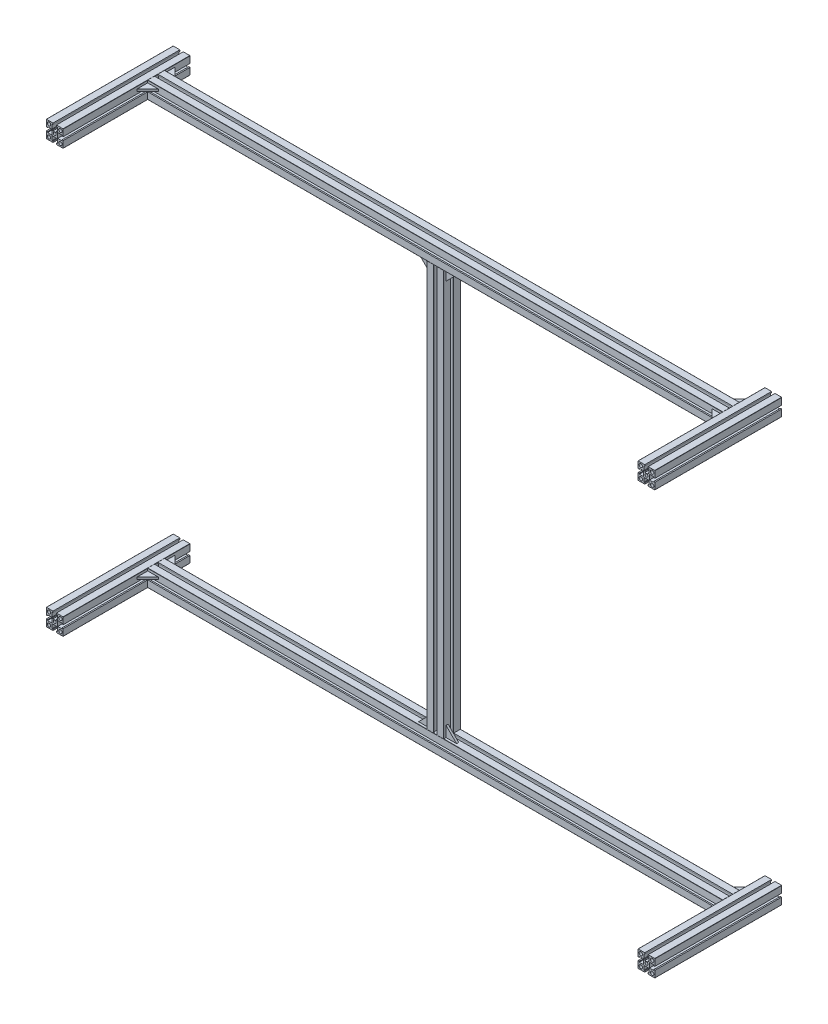
from build123d import *

# Parameters (mm, degrees)
SKETCH1_R                    = 3.4
SKETCH1_R_2                  = 4
F_40_X_40GF_X_R0_5_3_DEPTH   = 300
SKETCH1_ON_SEGMENT_2_R       = 3.4
SKETCH1_ON_SEGMENT_2_R_2     = 4
F_40_X_40GF_X_R0_5_3_2_DEPTH = 300
SKETCH1_ON_SEGMENT_3_R       = 3.4
SKETCH1_ON_SEGMENT_3_R_2     = 4
F_40_X_40GF_X_R0_5_3_3_DEPTH = 300
SKETCH1_ON_SEGMENT_4_R       = 3.4
SKETCH1_ON_SEGMENT_4_R_2     = 4
F_40_X_40GF_X_R0_5_3_4_DEPTH = 300
SKETCH1_ON_SEGMENT_5_R       = 3.4
SKETCH1_ON_SEGMENT_5_R_2     = 4
F_40_X_40GF_X_R0_5_3_5_DEPTH = 1402
SKETCH1_ON_SEGMENT_6_R       = 3.4
SKETCH1_ON_SEGMENT_6_R_2     = 4
F_40_X_40GF_X_R0_5_3_6_DEPTH = 1402
SKETCH1_ON_SEGMENT_7_R       = 3.4
SKETCH1_ON_SEGMENT_7_R_2     = 4
F_40_X_40GF_X_R0_5_3_7_DEPTH = 1002
GUSSET_2_THICKNESS           = 5
GUSSET_3_THICKNESS           = 5
GUSSET_4_THICKNESS           = 5
GUSSET_5_THICKNESS           = 5
GUSSET_6_THICKNESS           = 5
GUSSET_7_THICKNESS           = 5
GUSSET_8_THICKNESS           = 5
GUSSET_9_THICKNESS           = 5
GUSSET_12_THICKNESS          = 5
GUSSET_13_THICKNESS          = 5
GUSSET_14_THICKNESS          = 5
GUSSET_15_THICKNESS          = 5


with BuildPart() as part:
    # Sketch1 → 铝型材 40 X 40GF X R0.5(3) (new body)
    with BuildSketch(Plane(origin=(-700, 500, 0), x_dir=(1, 0, 0), z_dir=(0, 0, 1))):
        with BuildLine():
            Line((-19.5, 20), (-4, 20))
            Line((-4, 20), (-4, 17))
            Line((-4, 17), (-6, 17))
            Line((-6, 17), (-6, 7))
            Line((-6, 7), (-4, 7))
            Line((-4, 7), (-4, 4))
            Line((-4, 4), (4, 4))
            Line((4, 4), (4, 7))
            Line((4, 7), (6, 7))
            Line((6, 7), (6, 17))
            Line((6, 17), (4, 17))
            Line((4, 17), (4, 20))
            Line((4, 20), (19.5, 20))
            ThreePointArc((19.5, 20), (19.853553391, 19.853553391), (20, 19.5))
            Line((20, 19.5), (20, 4))
            Line((20, 4), (17, 4))
            Line((17, 4), (17, 6))
            Line((17, 6), (7, 6))
            Line((7, 6), (7, -6))
            Line((7, -6), (17, -6))
            Line((17, -6), (17, -4))
            Line((17, -4), (20, -4))
            Line((20, -4), (20, -19.5))
            ThreePointArc((20, -19.5), (19.853553391, -19.853553391), (19.5, -20))
            Line((19.5, -20), (4, -20))
            Line((4, -20), (4, -17))
            Line((4, -17), (6, -17))
            Line((6, -17), (6, -7))
            Line((6, -7), (-6, -7))
            Line((-6, -7), (-6, -17))
            Line((-6, -17), (-4, -17))
            Line((-4, -17), (-4, -20))
            Line((-4, -20), (-19.5, -20))
            ThreePointArc((-19.5, -20), (-19.853553391, -19.853553391), (-20, -19.5))
            Line((-20, -19.5), (-20, -4))
            Line((-20, -4), (-17, -4))
            Line((-17, -4), (-17, -6))
            Line((-17, -6), (-7, -6))
            Line((-7, -6), (-7, 6))
            Line((-7, 6), (-17, 6))
            Line((-17, 6), (-17, 4))
            Line((-17, 4), (-20, 4))
            Line((-20, 4), (-20, 19.5))
            ThreePointArc((-20, 19.5), (-19.853553391, 19.853553391), (-19.5, 20))
        make_face()
        Circle(SKETCH1_R, mode=Mode.SUBTRACT)
        with Locations((-13.435028843, 13.435028843)):
            Circle(SKETCH1_R_2, mode=Mode.SUBTRACT)
        with Locations((13.435028843, 13.435028843)):
            Circle(SKETCH1_R_2, mode=Mode.SUBTRACT)
        with Locations((13.435028843, -13.435028843)):
            Circle(SKETCH1_R_2, mode=Mode.SUBTRACT)
        with Locations((-13.435028843, -13.435028843)):
            Circle(SKETCH1_R_2, mode=Mode.SUBTRACT)
    extrude(amount=F_40_X_40GF_X_R0_5_3_DEPTH)


with BuildPart() as body_2:
    # Sketch1 on segment 2 (carried to segment 2) → 40 X 40GF X R0.5_3 2 (new body)
    with BuildSketch(Plane(origin=(700, 500, 0), x_dir=(1, 0, 0), z_dir=(0, 0, 1))):
        with BuildLine():
            Line((-19.5, 20), (-4, 20))
            Line((-4, 20), (-4, 17))
            Line((-4, 17), (-6, 17))
            Line((-6, 17), (-6, 7))
            Line((-6, 7), (-4, 7))
            Line((-4, 7), (-4, 4))
            Line((-4, 4), (4, 4))
            Line((4, 4), (4, 7))
            Line((4, 7), (6, 7))
            Line((6, 7), (6, 17))
            Line((6, 17), (4, 17))
            Line((4, 17), (4, 20))
            Line((4, 20), (19.5, 20))
            ThreePointArc((19.5, 20), (19.853553391, 19.853553391), (20, 19.5))
            Line((20, 19.5), (20, 4))
            Line((20, 4), (17, 4))
            Line((17, 4), (17, 6))
            Line((17, 6), (7, 6))
            Line((7, 6), (7, -6))
            Line((7, -6), (17, -6))
            Line((17, -6), (17, -4))
            Line((17, -4), (20, -4))
            Line((20, -4), (20, -19.5))
            ThreePointArc((20, -19.5), (19.853553391, -19.853553391), (19.5, -20))
            Line((19.5, -20), (4, -20))
            Line((4, -20), (4, -17))
            Line((4, -17), (6, -17))
            Line((6, -17), (6, -7))
            Line((6, -7), (-6, -7))
            Line((-6, -7), (-6, -17))
            Line((-6, -17), (-4, -17))
            Line((-4, -17), (-4, -20))
            Line((-4, -20), (-19.5, -20))
            ThreePointArc((-19.5, -20), (-19.853553391, -19.853553391), (-20, -19.5))
            Line((-20, -19.5), (-20, -4))
            Line((-20, -4), (-17, -4))
            Line((-17, -4), (-17, -6))
            Line((-17, -6), (-7, -6))
            Line((-7, -6), (-7, 6))
            Line((-7, 6), (-17, 6))
            Line((-17, 6), (-17, 4))
            Line((-17, 4), (-20, 4))
            Line((-20, 4), (-20, 19.5))
            ThreePointArc((-20, 19.5), (-19.853553391, 19.853553391), (-19.5, 20))
        make_face()
        Circle(SKETCH1_ON_SEGMENT_2_R, mode=Mode.SUBTRACT)
        with Locations((-13.435028843, 13.435028843)):
            Circle(SKETCH1_ON_SEGMENT_2_R_2, mode=Mode.SUBTRACT)
        with Locations((13.435028843, 13.435028843)):
            Circle(SKETCH1_ON_SEGMENT_2_R_2, mode=Mode.SUBTRACT)
        with Locations((13.435028843, -13.435028843)):
            Circle(SKETCH1_ON_SEGMENT_2_R_2, mode=Mode.SUBTRACT)
        with Locations((-13.435028843, -13.435028843)):
            Circle(SKETCH1_ON_SEGMENT_2_R_2, mode=Mode.SUBTRACT)
    extrude(amount=F_40_X_40GF_X_R0_5_3_2_DEPTH)


with BuildPart() as body_3:
    # Sketch1 on segment 3 (carried to segment 3) → 40 X 40GF X R0.5_3 3 (new body)
    with BuildSketch(Plane(origin=(700, -500, 0), x_dir=(1, 0, 0), z_dir=(0, 0, 1))):
        with BuildLine():
            Line((-19.5, 20), (-4, 20))
            Line((-4, 20), (-4, 17))
            Line((-4, 17), (-6, 17))
            Line((-6, 17), (-6, 7))
            Line((-6, 7), (-4, 7))
            Line((-4, 7), (-4, 4))
            Line((-4, 4), (4, 4))
            Line((4, 4), (4, 7))
            Line((4, 7), (6, 7))
            Line((6, 7), (6, 17))
            Line((6, 17), (4, 17))
            Line((4, 17), (4, 20))
            Line((4, 20), (19.5, 20))
            ThreePointArc((19.5, 20), (19.853553391, 19.853553391), (20, 19.5))
            Line((20, 19.5), (20, 4))
            Line((20, 4), (17, 4))
            Line((17, 4), (17, 6))
            Line((17, 6), (7, 6))
            Line((7, 6), (7, -6))
            Line((7, -6), (17, -6))
            Line((17, -6), (17, -4))
            Line((17, -4), (20, -4))
            Line((20, -4), (20, -19.5))
            ThreePointArc((20, -19.5), (19.853553391, -19.853553391), (19.5, -20))
            Line((19.5, -20), (4, -20))
            Line((4, -20), (4, -17))
            Line((4, -17), (6, -17))
            Line((6, -17), (6, -7))
            Line((6, -7), (-6, -7))
            Line((-6, -7), (-6, -17))
            Line((-6, -17), (-4, -17))
            Line((-4, -17), (-4, -20))
            Line((-4, -20), (-19.5, -20))
            ThreePointArc((-19.5, -20), (-19.853553391, -19.853553391), (-20, -19.5))
            Line((-20, -19.5), (-20, -4))
            Line((-20, -4), (-17, -4))
            Line((-17, -4), (-17, -6))
            Line((-17, -6), (-7, -6))
            Line((-7, -6), (-7, 6))
            Line((-7, 6), (-17, 6))
            Line((-17, 6), (-17, 4))
            Line((-17, 4), (-20, 4))
            Line((-20, 4), (-20, 19.5))
            ThreePointArc((-20, 19.5), (-19.853553391, 19.853553391), (-19.5, 20))
        make_face()
        Circle(SKETCH1_ON_SEGMENT_3_R, mode=Mode.SUBTRACT)
        with Locations((-13.435028843, 13.435028843)):
            Circle(SKETCH1_ON_SEGMENT_3_R_2, mode=Mode.SUBTRACT)
        with Locations((13.435028843, 13.435028843)):
            Circle(SKETCH1_ON_SEGMENT_3_R_2, mode=Mode.SUBTRACT)
        with Locations((13.435028843, -13.435028843)):
            Circle(SKETCH1_ON_SEGMENT_3_R_2, mode=Mode.SUBTRACT)
        with Locations((-13.435028843, -13.435028843)):
            Circle(SKETCH1_ON_SEGMENT_3_R_2, mode=Mode.SUBTRACT)
    extrude(amount=F_40_X_40GF_X_R0_5_3_3_DEPTH)


with BuildPart() as body_4:
    # Sketch1 on segment 4 (carried to segment 4) → 40 X 40GF X R0.5_3 4 (new body)
    with BuildSketch(Plane(origin=(-700, -500, 0), x_dir=(1, 0, 0), z_dir=(0, 0, 1))):
        with BuildLine():
            Line((-19.5, 20), (-4, 20))
            Line((-4, 20), (-4, 17))
            Line((-4, 17), (-6, 17))
            Line((-6, 17), (-6, 7))
            Line((-6, 7), (-4, 7))
            Line((-4, 7), (-4, 4))
            Line((-4, 4), (4, 4))
            Line((4, 4), (4, 7))
            Line((4, 7), (6, 7))
            Line((6, 7), (6, 17))
            Line((6, 17), (4, 17))
            Line((4, 17), (4, 20))
            Line((4, 20), (19.5, 20))
            ThreePointArc((19.5, 20), (19.853553391, 19.853553391), (20, 19.5))
            Line((20, 19.5), (20, 4))
            Line((20, 4), (17, 4))
            Line((17, 4), (17, 6))
            Line((17, 6), (7, 6))
            Line((7, 6), (7, -6))
            Line((7, -6), (17, -6))
            Line((17, -6), (17, -4))
            Line((17, -4), (20, -4))
            Line((20, -4), (20, -19.5))
            ThreePointArc((20, -19.5), (19.853553391, -19.853553391), (19.5, -20))
            Line((19.5, -20), (4, -20))
            Line((4, -20), (4, -17))
            Line((4, -17), (6, -17))
            Line((6, -17), (6, -7))
            Line((6, -7), (-6, -7))
            Line((-6, -7), (-6, -17))
            Line((-6, -17), (-4, -17))
            Line((-4, -17), (-4, -20))
            Line((-4, -20), (-19.5, -20))
            ThreePointArc((-19.5, -20), (-19.853553391, -19.853553391), (-20, -19.5))
            Line((-20, -19.5), (-20, -4))
            Line((-20, -4), (-17, -4))
            Line((-17, -4), (-17, -6))
            Line((-17, -6), (-7, -6))
            Line((-7, -6), (-7, 6))
            Line((-7, 6), (-17, 6))
            Line((-17, 6), (-17, 4))
            Line((-17, 4), (-20, 4))
            Line((-20, 4), (-20, 19.5))
            ThreePointArc((-20, 19.5), (-19.853553391, 19.853553391), (-19.5, 20))
        make_face()
        Circle(SKETCH1_ON_SEGMENT_4_R, mode=Mode.SUBTRACT)
        with Locations((-13.435028843, 13.435028843)):
            Circle(SKETCH1_ON_SEGMENT_4_R_2, mode=Mode.SUBTRACT)
        with Locations((13.435028843, 13.435028843)):
            Circle(SKETCH1_ON_SEGMENT_4_R_2, mode=Mode.SUBTRACT)
        with Locations((13.435028843, -13.435028843)):
            Circle(SKETCH1_ON_SEGMENT_4_R_2, mode=Mode.SUBTRACT)
        with Locations((-13.435028843, -13.435028843)):
            Circle(SKETCH1_ON_SEGMENT_4_R_2, mode=Mode.SUBTRACT)
    extrude(amount=F_40_X_40GF_X_R0_5_3_4_DEPTH)


with BuildPart() as body_5:
    # Sketch1 on segment 5 (carried to segment 5) → 40 X 40GF X R0.5_3 5 (new body)
    with BuildSketch(Plane(origin=(-701, 500, 80), x_dir=(0, 0, -1), z_dir=(1, 0, 0))):
        with BuildLine():
            Line((-19.5, 20), (-4, 20))
            Line((-4, 20), (-4, 17))
            Line((-4, 17), (-6, 17))
            Line((-6, 17), (-6, 7))
            Line((-6, 7), (-4, 7))
            Line((-4, 7), (-4, 4))
            Line((-4, 4), (4, 4))
            Line((4, 4), (4, 7))
            Line((4, 7), (6, 7))
            Line((6, 7), (6, 17))
            Line((6, 17), (4, 17))
            Line((4, 17), (4, 20))
            Line((4, 20), (19.5, 20))
            ThreePointArc((19.5, 20), (19.853553391, 19.853553391), (20, 19.5))
            Line((20, 19.5), (20, 4))
            Line((20, 4), (17, 4))
            Line((17, 4), (17, 6))
            Line((17, 6), (7, 6))
            Line((7, 6), (7, -6))
            Line((7, -6), (17, -6))
            Line((17, -6), (17, -4))
            Line((17, -4), (20, -4))
            Line((20, -4), (20, -19.5))
            ThreePointArc((20, -19.5), (19.853553391, -19.853553391), (19.5, -20))
            Line((19.5, -20), (4, -20))
            Line((4, -20), (4, -17))
            Line((4, -17), (6, -17))
            Line((6, -17), (6, -7))
            Line((6, -7), (-6, -7))
            Line((-6, -7), (-6, -17))
            Line((-6, -17), (-4, -17))
            Line((-4, -17), (-4, -20))
            Line((-4, -20), (-19.5, -20))
            ThreePointArc((-19.5, -20), (-19.853553391, -19.853553391), (-20, -19.5))
            Line((-20, -19.5), (-20, -4))
            Line((-20, -4), (-17, -4))
            Line((-17, -4), (-17, -6))
            Line((-17, -6), (-7, -6))
            Line((-7, -6), (-7, 6))
            Line((-7, 6), (-17, 6))
            Line((-17, 6), (-17, 4))
            Line((-17, 4), (-20, 4))
            Line((-20, 4), (-20, 19.5))
            ThreePointArc((-20, 19.5), (-19.853553391, 19.853553391), (-19.5, 20))
        make_face()
        Circle(SKETCH1_ON_SEGMENT_5_R, mode=Mode.SUBTRACT)
        with Locations((-13.435028843, 13.435028843)):
            Circle(SKETCH1_ON_SEGMENT_5_R_2, mode=Mode.SUBTRACT)
        with Locations((13.435028843, 13.435028843)):
            Circle(SKETCH1_ON_SEGMENT_5_R_2, mode=Mode.SUBTRACT)
        with Locations((13.435028843, -13.435028843)):
            Circle(SKETCH1_ON_SEGMENT_5_R_2, mode=Mode.SUBTRACT)
        with Locations((-13.435028843, -13.435028843)):
            Circle(SKETCH1_ON_SEGMENT_5_R_2, mode=Mode.SUBTRACT)
    extrude(amount=F_40_X_40GF_X_R0_5_3_5_DEPTH)

    # 40 X 40GF X R0.5_3 5 end butt 1
    split(bisect_by=Plane(origin=(-680, 500, 80), x_dir=(0, 1, 0), z_dir=(1, 0, 0)), keep=Keep.TOP)

    # 40 X 40GF X R0.5_3 5 end butt 2
    split(bisect_by=Plane(origin=(680, 500, 80), x_dir=(0, -1, 0), z_dir=(-1, 0, 0)), keep=Keep.TOP)


with BuildPart() as body_6:
    # Sketch1 on segment 6 (carried to segment 6) → 40 X 40GF X R0.5_3 6 (new body)
    with BuildSketch(Plane(origin=(701, -500, 80), x_dir=(0, 0, 1), z_dir=(-1, 0, 0))):
        with BuildLine():
            Line((-19.5, 20), (-4, 20))
            Line((-4, 20), (-4, 17))
            Line((-4, 17), (-6, 17))
            Line((-6, 17), (-6, 7))
            Line((-6, 7), (-4, 7))
            Line((-4, 7), (-4, 4))
            Line((-4, 4), (4, 4))
            Line((4, 4), (4, 7))
            Line((4, 7), (6, 7))
            Line((6, 7), (6, 17))
            Line((6, 17), (4, 17))
            Line((4, 17), (4, 20))
            Line((4, 20), (19.5, 20))
            ThreePointArc((19.5, 20), (19.853553391, 19.853553391), (20, 19.5))
            Line((20, 19.5), (20, 4))
            Line((20, 4), (17, 4))
            Line((17, 4), (17, 6))
            Line((17, 6), (7, 6))
            Line((7, 6), (7, -6))
            Line((7, -6), (17, -6))
            Line((17, -6), (17, -4))
            Line((17, -4), (20, -4))
            Line((20, -4), (20, -19.5))
            ThreePointArc((20, -19.5), (19.853553391, -19.853553391), (19.5, -20))
            Line((19.5, -20), (4, -20))
            Line((4, -20), (4, -17))
            Line((4, -17), (6, -17))
            Line((6, -17), (6, -7))
            Line((6, -7), (-6, -7))
            Line((-6, -7), (-6, -17))
            Line((-6, -17), (-4, -17))
            Line((-4, -17), (-4, -20))
            Line((-4, -20), (-19.5, -20))
            ThreePointArc((-19.5, -20), (-19.853553391, -19.853553391), (-20, -19.5))
            Line((-20, -19.5), (-20, -4))
            Line((-20, -4), (-17, -4))
            Line((-17, -4), (-17, -6))
            Line((-17, -6), (-7, -6))
            Line((-7, -6), (-7, 6))
            Line((-7, 6), (-17, 6))
            Line((-17, 6), (-17, 4))
            Line((-17, 4), (-20, 4))
            Line((-20, 4), (-20, 19.5))
            ThreePointArc((-20, 19.5), (-19.853553391, 19.853553391), (-19.5, 20))
        make_face()
        Circle(SKETCH1_ON_SEGMENT_6_R, mode=Mode.SUBTRACT)
        with Locations((-13.435028843, 13.435028843)):
            Circle(SKETCH1_ON_SEGMENT_6_R_2, mode=Mode.SUBTRACT)
        with Locations((13.435028843, 13.435028843)):
            Circle(SKETCH1_ON_SEGMENT_6_R_2, mode=Mode.SUBTRACT)
        with Locations((13.435028843, -13.435028843)):
            Circle(SKETCH1_ON_SEGMENT_6_R_2, mode=Mode.SUBTRACT)
        with Locations((-13.435028843, -13.435028843)):
            Circle(SKETCH1_ON_SEGMENT_6_R_2, mode=Mode.SUBTRACT)
    extrude(amount=F_40_X_40GF_X_R0_5_3_6_DEPTH)

    # 40 X 40GF X R0.5_3 6 end butt 1
    split(bisect_by=Plane(origin=(680, -500, 80), x_dir=(0, -1, 0), z_dir=(-1, 0, 0)), keep=Keep.TOP)

    # 40 X 40GF X R0.5_3 6 end butt 2
    split(bisect_by=Plane(origin=(-680, -500, 80), x_dir=(0, 1, 0), z_dir=(1, 0, 0)), keep=Keep.TOP)


with BuildPart() as body_7:
    # Sketch1 on segment 7 (carried to segment 7) → 40 X 40GF X R0.5_3 7 (new body)
    with BuildSketch(Plane(origin=(0, 501, 80), x_dir=(1, 0, 0), z_dir=(0, -1, 0))):
        with BuildLine():
            Line((-19.5, 20), (-4, 20))
            Line((-4, 20), (-4, 17))
            Line((-4, 17), (-6, 17))
            Line((-6, 17), (-6, 7))
            Line((-6, 7), (-4, 7))
            Line((-4, 7), (-4, 4))
            Line((-4, 4), (4, 4))
            Line((4, 4), (4, 7))
            Line((4, 7), (6, 7))
            Line((6, 7), (6, 17))
            Line((6, 17), (4, 17))
            Line((4, 17), (4, 20))
            Line((4, 20), (19.5, 20))
            ThreePointArc((19.5, 20), (19.853553391, 19.853553391), (20, 19.5))
            Line((20, 19.5), (20, 4))
            Line((20, 4), (17, 4))
            Line((17, 4), (17, 6))
            Line((17, 6), (7, 6))
            Line((7, 6), (7, -6))
            Line((7, -6), (17, -6))
            Line((17, -6), (17, -4))
            Line((17, -4), (20, -4))
            Line((20, -4), (20, -19.5))
            ThreePointArc((20, -19.5), (19.853553391, -19.853553391), (19.5, -20))
            Line((19.5, -20), (4, -20))
            Line((4, -20), (4, -17))
            Line((4, -17), (6, -17))
            Line((6, -17), (6, -7))
            Line((6, -7), (-6, -7))
            Line((-6, -7), (-6, -17))
            Line((-6, -17), (-4, -17))
            Line((-4, -17), (-4, -20))
            Line((-4, -20), (-19.5, -20))
            ThreePointArc((-19.5, -20), (-19.853553391, -19.853553391), (-20, -19.5))
            Line((-20, -19.5), (-20, -4))
            Line((-20, -4), (-17, -4))
            Line((-17, -4), (-17, -6))
            Line((-17, -6), (-7, -6))
            Line((-7, -6), (-7, 6))
            Line((-7, 6), (-17, 6))
            Line((-17, 6), (-17, 4))
            Line((-17, 4), (-20, 4))
            Line((-20, 4), (-20, 19.5))
            ThreePointArc((-20, 19.5), (-19.853553391, 19.853553391), (-19.5, 20))
        make_face()
        Circle(SKETCH1_ON_SEGMENT_7_R, mode=Mode.SUBTRACT)
        with Locations((-13.435028843, 13.435028843)):
            Circle(SKETCH1_ON_SEGMENT_7_R_2, mode=Mode.SUBTRACT)
        with Locations((13.435028843, 13.435028843)):
            Circle(SKETCH1_ON_SEGMENT_7_R_2, mode=Mode.SUBTRACT)
        with Locations((13.435028843, -13.435028843)):
            Circle(SKETCH1_ON_SEGMENT_7_R_2, mode=Mode.SUBTRACT)
        with Locations((-13.435028843, -13.435028843)):
            Circle(SKETCH1_ON_SEGMENT_7_R_2, mode=Mode.SUBTRACT)
    extrude(amount=F_40_X_40GF_X_R0_5_3_7_DEPTH)

    # 40 X 40GF X R0.5_3 7 end butt 1
    split(bisect_by=Plane(origin=(0, 480, 80), x_dir=(1, 0, 0), z_dir=(0, -1, 0)), keep=Keep.TOP)

    # 40 X 40GF X R0.5_3 7 end butt 2
    split(bisect_by=Plane(origin=(0, -480, 80), x_dir=(-1, 0, 0), z_dir=(0, 1, 0)), keep=Keep.TOP)


with BuildPart() as body_8:
    # Gusset 2: a gusset: a plate 5.0 thick in the corner of two members, its outline drawn in place
    gusset_2_outline = Wire([Line((680, 509.25, 100), (680, 509.25, 125)), Line((680, 509.25, 125), (655, 509.25, 100)), Line((655, 509.25, 100), (680, 509.25, 100))])
    add(extrude(Face(gusset_2_outline), amount=GUSSET_2_THICKNESS, dir=(0, 1, 0)))


with BuildPart() as body_9:
    # Gusset 3: a gusset: a plate 5.0 thick in the corner of two members, its outline drawn in place
    gusset_3_outline = Wire([Line((680, 509.25, 60), (655, 509.25, 60)), Line((655, 509.25, 60), (680, 509.25, 35)), Line((680, 509.25, 35), (680, 509.25, 60))])
    add(extrude(Face(gusset_3_outline), amount=GUSSET_3_THICKNESS, dir=(0, 1, 0)))


with BuildPart() as body_10:
    # Gusset 4: a gusset: a plate 5.0 thick in the corner of two members, its outline drawn in place
    gusset_4_outline = Wire([Line((-20, 480, 89.25), (-20, 455, 89.25)), Line((-20, 455, 89.25), (-45, 480, 89.25)), Line((-45, 480, 89.25), (-20, 480, 89.25))])
    add(extrude(Face(gusset_4_outline), amount=GUSSET_4_THICKNESS, dir=(0, 0, 1)))


with BuildPart() as body_11:
    # Gusset 5: a gusset: a plate 5.0 thick in the corner of two members, its outline drawn in place
    gusset_5_outline = Wire([Line((20, 480, 89.25), (45, 480, 89.25)), Line((45, 480, 89.25), (20, 455, 89.25)), Line((20, 455, 89.25), (20, 480, 89.25))])
    add(extrude(Face(gusset_5_outline), amount=GUSSET_5_THICKNESS, dir=(0, 0, 1)))


with BuildPart() as body_12:
    # Gusset 6: a gusset: a plate 5.0 thick in the corner of two members, its outline drawn in place
    gusset_6_outline = Wire([Line((-20, -480, 94.25), (-20, -455, 94.25)), Line((-20, -455, 94.25), (-45, -480, 94.25)), Line((-45, -480, 94.25), (-20, -480, 94.25))])
    add(extrude(Face(gusset_6_outline), amount=GUSSET_6_THICKNESS, dir=(0, 0, -1)))


with BuildPart() as body_13:
    # Gusset 7: a gusset: a plate 5.0 thick in the corner of two members, its outline drawn in place
    gusset_7_outline = Wire([Line((20, -480, 94.25), (45, -480, 94.25)), Line((45, -480, 94.25), (20, -455, 94.25)), Line((20, -455, 94.25), (20, -480, 94.25))])
    add(extrude(Face(gusset_7_outline), amount=GUSSET_7_THICKNESS, dir=(0, 0, -1)))


with BuildPart() as body_14:
    # Gusset 8: a gusset: a plate 5.0 thick in the corner of two members, its outline drawn in place
    gusset_8_outline = Wire([Line((-680, 509.25, 100), (-655, 509.25, 100)), Line((-655, 509.25, 100), (-680, 509.25, 125)), Line((-680, 509.25, 125), (-680, 509.25, 100))])
    add(extrude(Face(gusset_8_outline), amount=GUSSET_8_THICKNESS, dir=(0, 1, 0)))


with BuildPart() as body_15:
    # Gusset 9: a gusset: a plate 5.0 thick in the corner of two members, its outline drawn in place
    gusset_9_outline = Wire([Line((-680, 514.25, 60), (-655, 514.25, 60)), Line((-655, 514.25, 60), (-680, 514.25, 35)), Line((-680, 514.25, 35), (-680, 514.25, 60))])
    add(extrude(Face(gusset_9_outline), amount=GUSSET_9_THICKNESS, dir=(0, -1, 0)))


with BuildPart() as body_16:
    # Gusset 12: a gusset: a plate 5.0 thick in the corner of two members, its outline drawn in place
    gusset_12_outline = Wire([Line((680, -485.75, 60), (680, -485.75, 35)), Line((680, -485.75, 35), (655, -485.75, 60)), Line((655, -485.75, 60), (680, -485.75, 60))])
    add(extrude(Face(gusset_12_outline), amount=GUSSET_12_THICKNESS, dir=(0, -1, 0)))


with BuildPart() as body_17:
    # Gusset 13: a gusset: a plate 5.0 thick in the corner of two members, its outline drawn in place
    gusset_13_outline = Wire([Line((680, -514.25, 100), (680, -514.25, 125)), Line((680, -514.25, 125), (655, -514.25, 100)), Line((655, -514.25, 100), (680, -514.25, 100))])
    add(extrude(Face(gusset_13_outline), amount=GUSSET_13_THICKNESS, dir=(0, 1, 0)))


with BuildPart() as body_18:
    # Gusset 14: a gusset: a plate 5.0 thick in the corner of two members, its outline drawn in place
    gusset_14_outline = Wire([Line((-680, -485.75, 60), (-655, -485.75, 60)), Line((-655, -485.75, 60), (-680, -485.75, 35)), Line((-680, -485.75, 35), (-680, -485.75, 60))])
    add(extrude(Face(gusset_14_outline), amount=GUSSET_14_THICKNESS, dir=(0, -1, 0)))


with BuildPart() as body_19:
    # Gusset 15: a gusset: a plate 5.0 thick in the corner of two members, its outline drawn in place
    gusset_15_outline = Wire([Line((-680, -485.75, 100), (-680, -485.75, 125)), Line((-680, -485.75, 125), (-655, -485.75, 100)), Line((-655, -485.75, 100), (-680, -485.75, 100))])
    add(extrude(Face(gusset_15_outline), amount=GUSSET_15_THICKNESS, dir=(0, -1, 0)))


solid = Compound([part.part, body_2.part, body_3.part, body_4.part, body_5.part, body_6.part, body_7.part, body_8.part, body_9.part, body_10.part, body_11.part, body_12.part, body_13.part, body_14.part, body_15.part, body_16.part, body_17.part, body_18.part, body_19.part])
